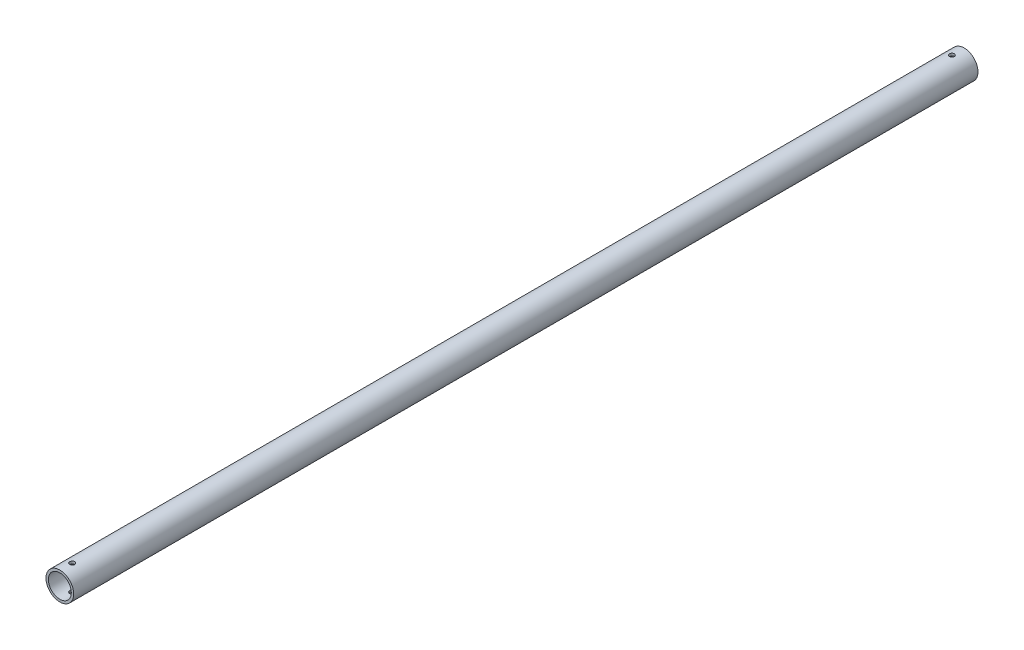
from build123d import *

# Parameters (mm, degrees)
SKETCH_1_R          = 16.85
SKETCH_1_R_2        = 13.95
EXTRUDE_1_DEPTH     = 1100
SKETCH_2_R          = 3
CUT_EXTRUDE_1_DEPTH = 16.85


with BuildPart() as part:
    # 草图1 → 凸台-拉伸1 (new body)
    with BuildSketch(Plane.XY):
        Circle(SKETCH_1_R)
        Circle(SKETCH_1_R_2, mode=Mode.SUBTRACT)
    extrude(amount=EXTRUDE_1_DEPTH)

    # 草图2 → 切除-拉伸1 (cut, symmetric)
    with BuildSketch(Plane(origin=(0, 0, 0), x_dir=(1, 0, 0), z_dir=(0, 1, 0))):
        with Locations(Location((0, -15, 0), (0, 0, 270))):
            Circle(SKETCH_2_R)
        with Locations(Location((0, -1085, 0), (0, 0, 270))):
            Circle(SKETCH_2_R)
    extrude(amount=CUT_EXTRUDE_1_DEPTH, both=True, mode=Mode.SUBTRACT)


solid = part.part
